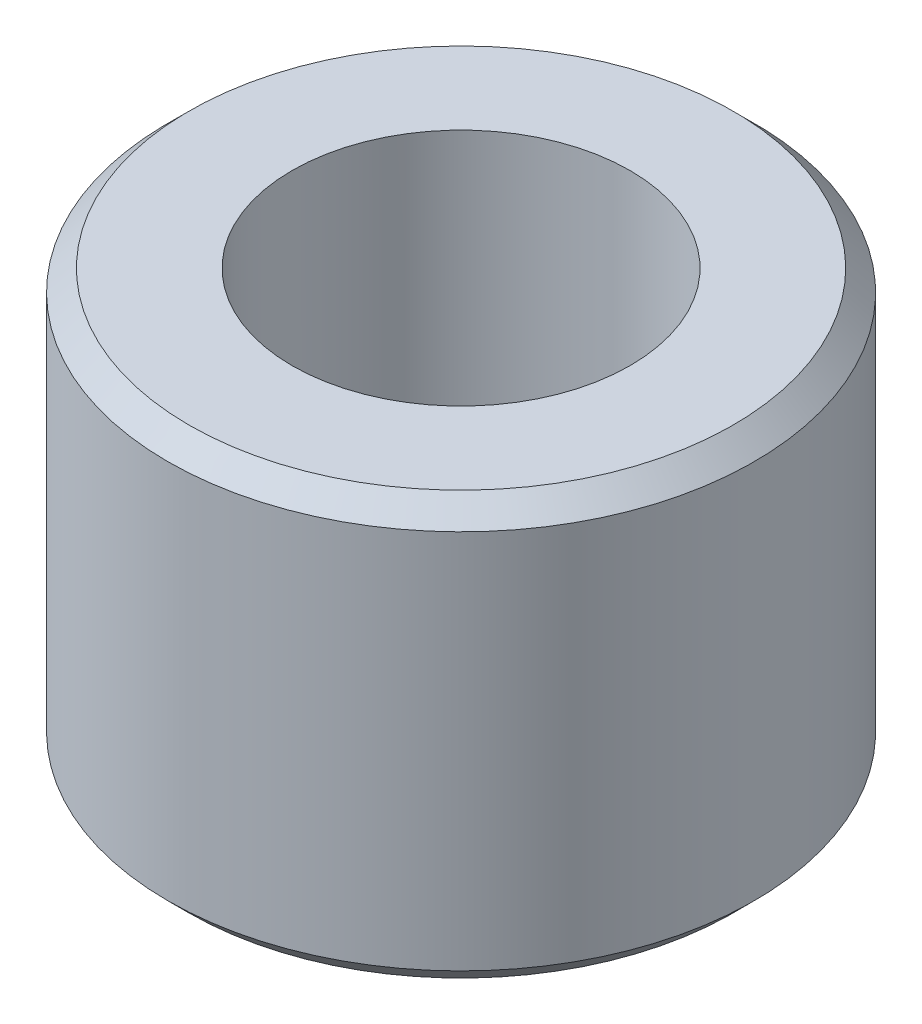
from build123d import *

# Parameters (mm, degrees)
SKETCH_1_R      = 27.75
SKETCH_1_R_2    = 16
EXTRUDE_1_DEPTH = 40
CHAMFER_1_SIZE  = 2
SKETCH_2_R      = 16
SKETCH_2_R_2    = 7.5
EXTRUDE_2_DEPTH = 5


with BuildPart() as part:
    # 草图1 → 凸台-拉伸1 (new body)
    with BuildSketch(Plane(origin=(0, 0, 0), x_dir=(1, 0, 0), z_dir=(0, 1, 0))):
        with Locations(Location((0, 0, 0), (0, 0, 270))):
            Circle(SKETCH_1_R)
        with Locations(Location((0, 0, 0), (0, 0, 270))):
            Circle(SKETCH_1_R_2, mode=Mode.SUBTRACT)
    extrude(amount=EXTRUDE_1_DEPTH)

    # 倒角1
    chamfer_1_edges = [part.edges().sort_by_distance(p)[0] for p in [
        (0, 0, -27.75),
        (0, 40, -27.75),
    ]]
    chamfer(chamfer_1_edges, length=CHAMFER_1_SIZE)

    # 草图2 → 凸台-拉伸2 (add)
    with BuildSketch(Plane.XZ):
        with Locations(Location((0, 0, 0), (0, 0, 270))):
            Circle(SKETCH_2_R)
        with Locations(Location((0, 0, 0), (0, 0, 270))):
            Circle(SKETCH_2_R_2, mode=Mode.SUBTRACT)
    extrude(amount=-EXTRUDE_2_DEPTH)


solid = part.part
